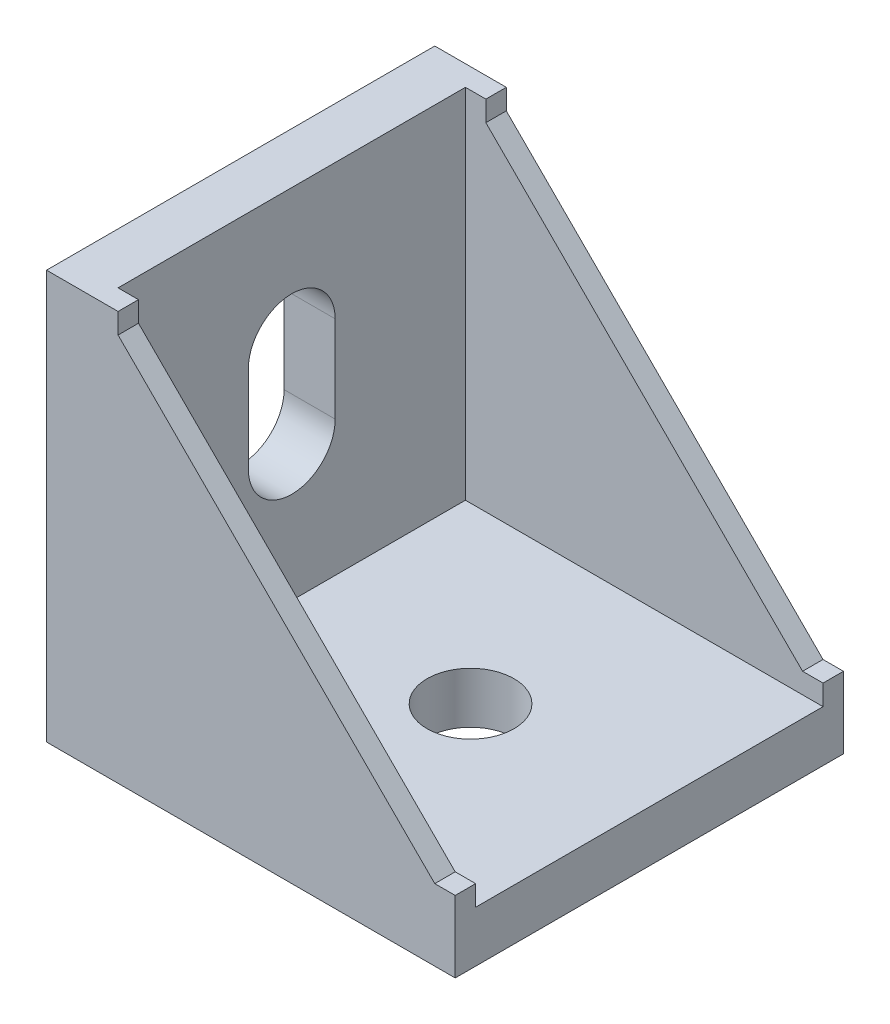
SolidWorks part; units mm, degrees
ref_plane "Front Plane" through (0, 0, 0) normal (0, 0, 1) x (1, 0, 0)
ref_plane "Top Plane" through (0, 0, 0) normal (0, 1, 0) x (1, 0, 0)
ref_plane "Right Plane" through (0, 0, 0) normal (1, 0, 0) x (0, 0, -1)
sketch "Sketch1" plane through (0, 0, 0) normal (0, 0, 1) x (1, 0, 0)
  line L0 (0, 0) -> (40, 0)
  line L1 (0, 0) -> (0, 40)
  line L2 (5, 5) -> (40, 5)
  line L3 (5, 5) -> (5, 40)
  line L4 (0, 40) -> (5, 40)
  line L5 (40, 5) -> (40, 0)
  dimension "D1" = 5
extrude "Boss-Extrude1" add sketch "Sketch1" along normal blind 38
sketch "Sketch2" plane through (0, 0, 38) normal (0, 0, 1) x (1, 0, 0)
  line L0 (7, 40) -> (7, 38)
  line L1 (7, 38) -> (38, 7)
  line L2 (5, 40) -> (7, 40)
  line L3 (40, 7) -> (40, 5)
  line L4 (38, 7) -> (40, 7)
  line L6 (0, 40) -> (0, 0)
  line L7 (0, 0) -> (40, 0)
  line L8 (40, 0) -> (40, 5)
  line L9 (40, 5) -> (5, 5)
  line L10 (5, 5) -> (5, 40)
  line L11 (5, 40) -> (0, 40)
  line L15 (40, 5) -> (5, 5)
  line L16 (5, 5) -> (5, 40)
  dimension "D3" = 2
  dimension "D2" = 2
  dimension "D4" = 2
  dimension "D5" = 2
  dimension "D1" = 0
extrude "Boss-Extrude2" add sketch "Sketch2" against normal blind 2
sketch "Sketch3" plane through (0, 0, 0) normal (0, 0, -1) x (-1, 0, 0)
  line L0 (-38, 7) -> (-7, 38) construction
  line L1 (-7, 38) -> (-7, 40) construction
  line L2 (-7, 40) -> (-5, 40) construction
  line L3 (-5, 5) -> (-5, 40) construction
  line L4 (-40, 5) -> (-40, 7) construction
  line L5 (-40, 7) -> (-38, 7) construction
  line L6 (0, 0) -> (0, 40)
  line L7 (0, 40) -> (-5, 40)
  line L8 (-5, 40) -> (-5, 5)
  line L9 (-5, 5) -> (-40, 5)
  line L10 (-40, 5) -> (-40, 0)
  line L11 (-40, 0) -> (0, 0)
  line L12 (-38, 7) -> (-7, 38)
  line L13 (-7, 38) -> (-7, 40)
  line L14 (-7, 40) -> (-5, 40)
  line L15 (-5, 5) -> (-40, 5)
  line L16 (-5, 5) -> (-5, 40)
  line L17 (-40, 5) -> (-40, 7)
  line L18 (-40, 7) -> (-38, 7)
  dimension "D1" = 0
extrude "Boss-Extrude3" add sketch "Sketch3" against normal blind 2
sketch "Sketch4" plane through (0, 5, 0) normal (0, 1, 0) x (1, 0, 0)
  line L0 (22.5, -36) -> (22.5, -2) construction
  line L1 (5, -36) -> (5, -2) construction
  line L2 (40, -38) -> (40, 0) construction
  line L4 (5, -36) -> (40, -36) construction
  line L5 (40, -2) -> (5, -2) construction
  line L6 (5, -19) -> (40, -19) construction
  circle A0 centre (22.5, -19) radius 4.25
extrude "Cut-Extrude1" cut sketch "Sketch4" against normal through all
sketch "Sketch5" plane through (0, 0, 0) normal (-1, 0, 0) x (0, 0, 1)
  line L0 (19, 40) -> (19, 5) construction
  line L1 (38, 40) -> (0, 40) construction
  line L2 (36, 5) -> (2, 5) construction
  line L3 (36, 22.5) -> (2, 22.5) construction
  line L4 (36, 40) -> (36, 5) construction
  line L5 (2, 5) -> (2, 40) construction
  line L6 (14.75, 22.5) -> (14.75, 18.25)
  line L8 (23.25, 18.25) -> (23.25, 26.75)
  line L10 (14.75, 26.75) -> (14.75, 22.5)
  arc A1 (23.25, 26.75) -> (14.75, 26.75) centre (19, 26.75) ccw
  arc A2 (14.75, 18.25) -> (23.25, 18.25) centre (19, 18.25) ccw
extrude "Cut-Extrude2" cut sketch "Sketch5" against normal through all
